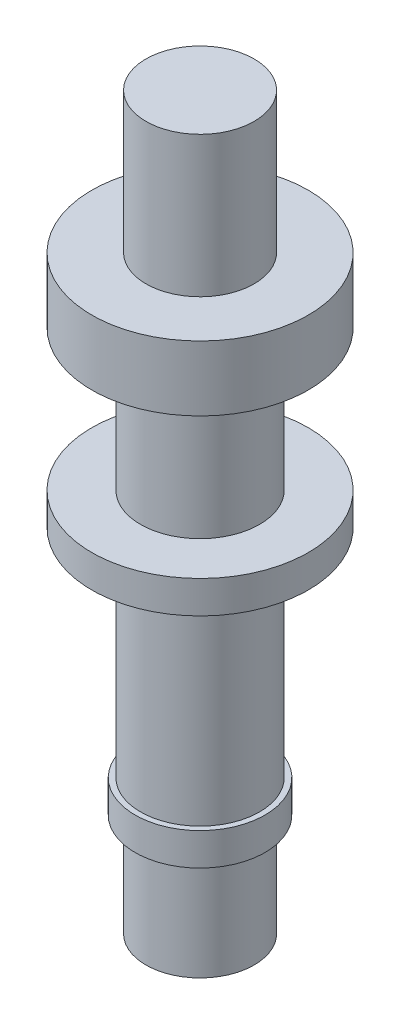
from build123d import *


with BuildPart() as part:
    # 草图1 → 旋转1 (revolve)
    with BuildSketch(Plane.XY, mode=Mode.PRIVATE) as revolve_1_sk:
        Polygon((0, 0), (5, 0), (5, 9.5), (6, 9.5), (6, 12.5), (5.5, 12.5), (5.5, 32.5), (10, 32.5), (10, 35.5), (5.5, 35.5), (5.5, 48.5), (10, 48.5), (10, 54.5), (5, 54.5), (5, 67.5), (0, 67.5), align=None)
    revolve(revolve_1_sk.sketch.rotate(Axis((0, -28.718438831, 0), (0, 1, 0)), 90), axis=Axis((0, -28.718438831, 0), (0, 1, 0)))


solid = part.part
